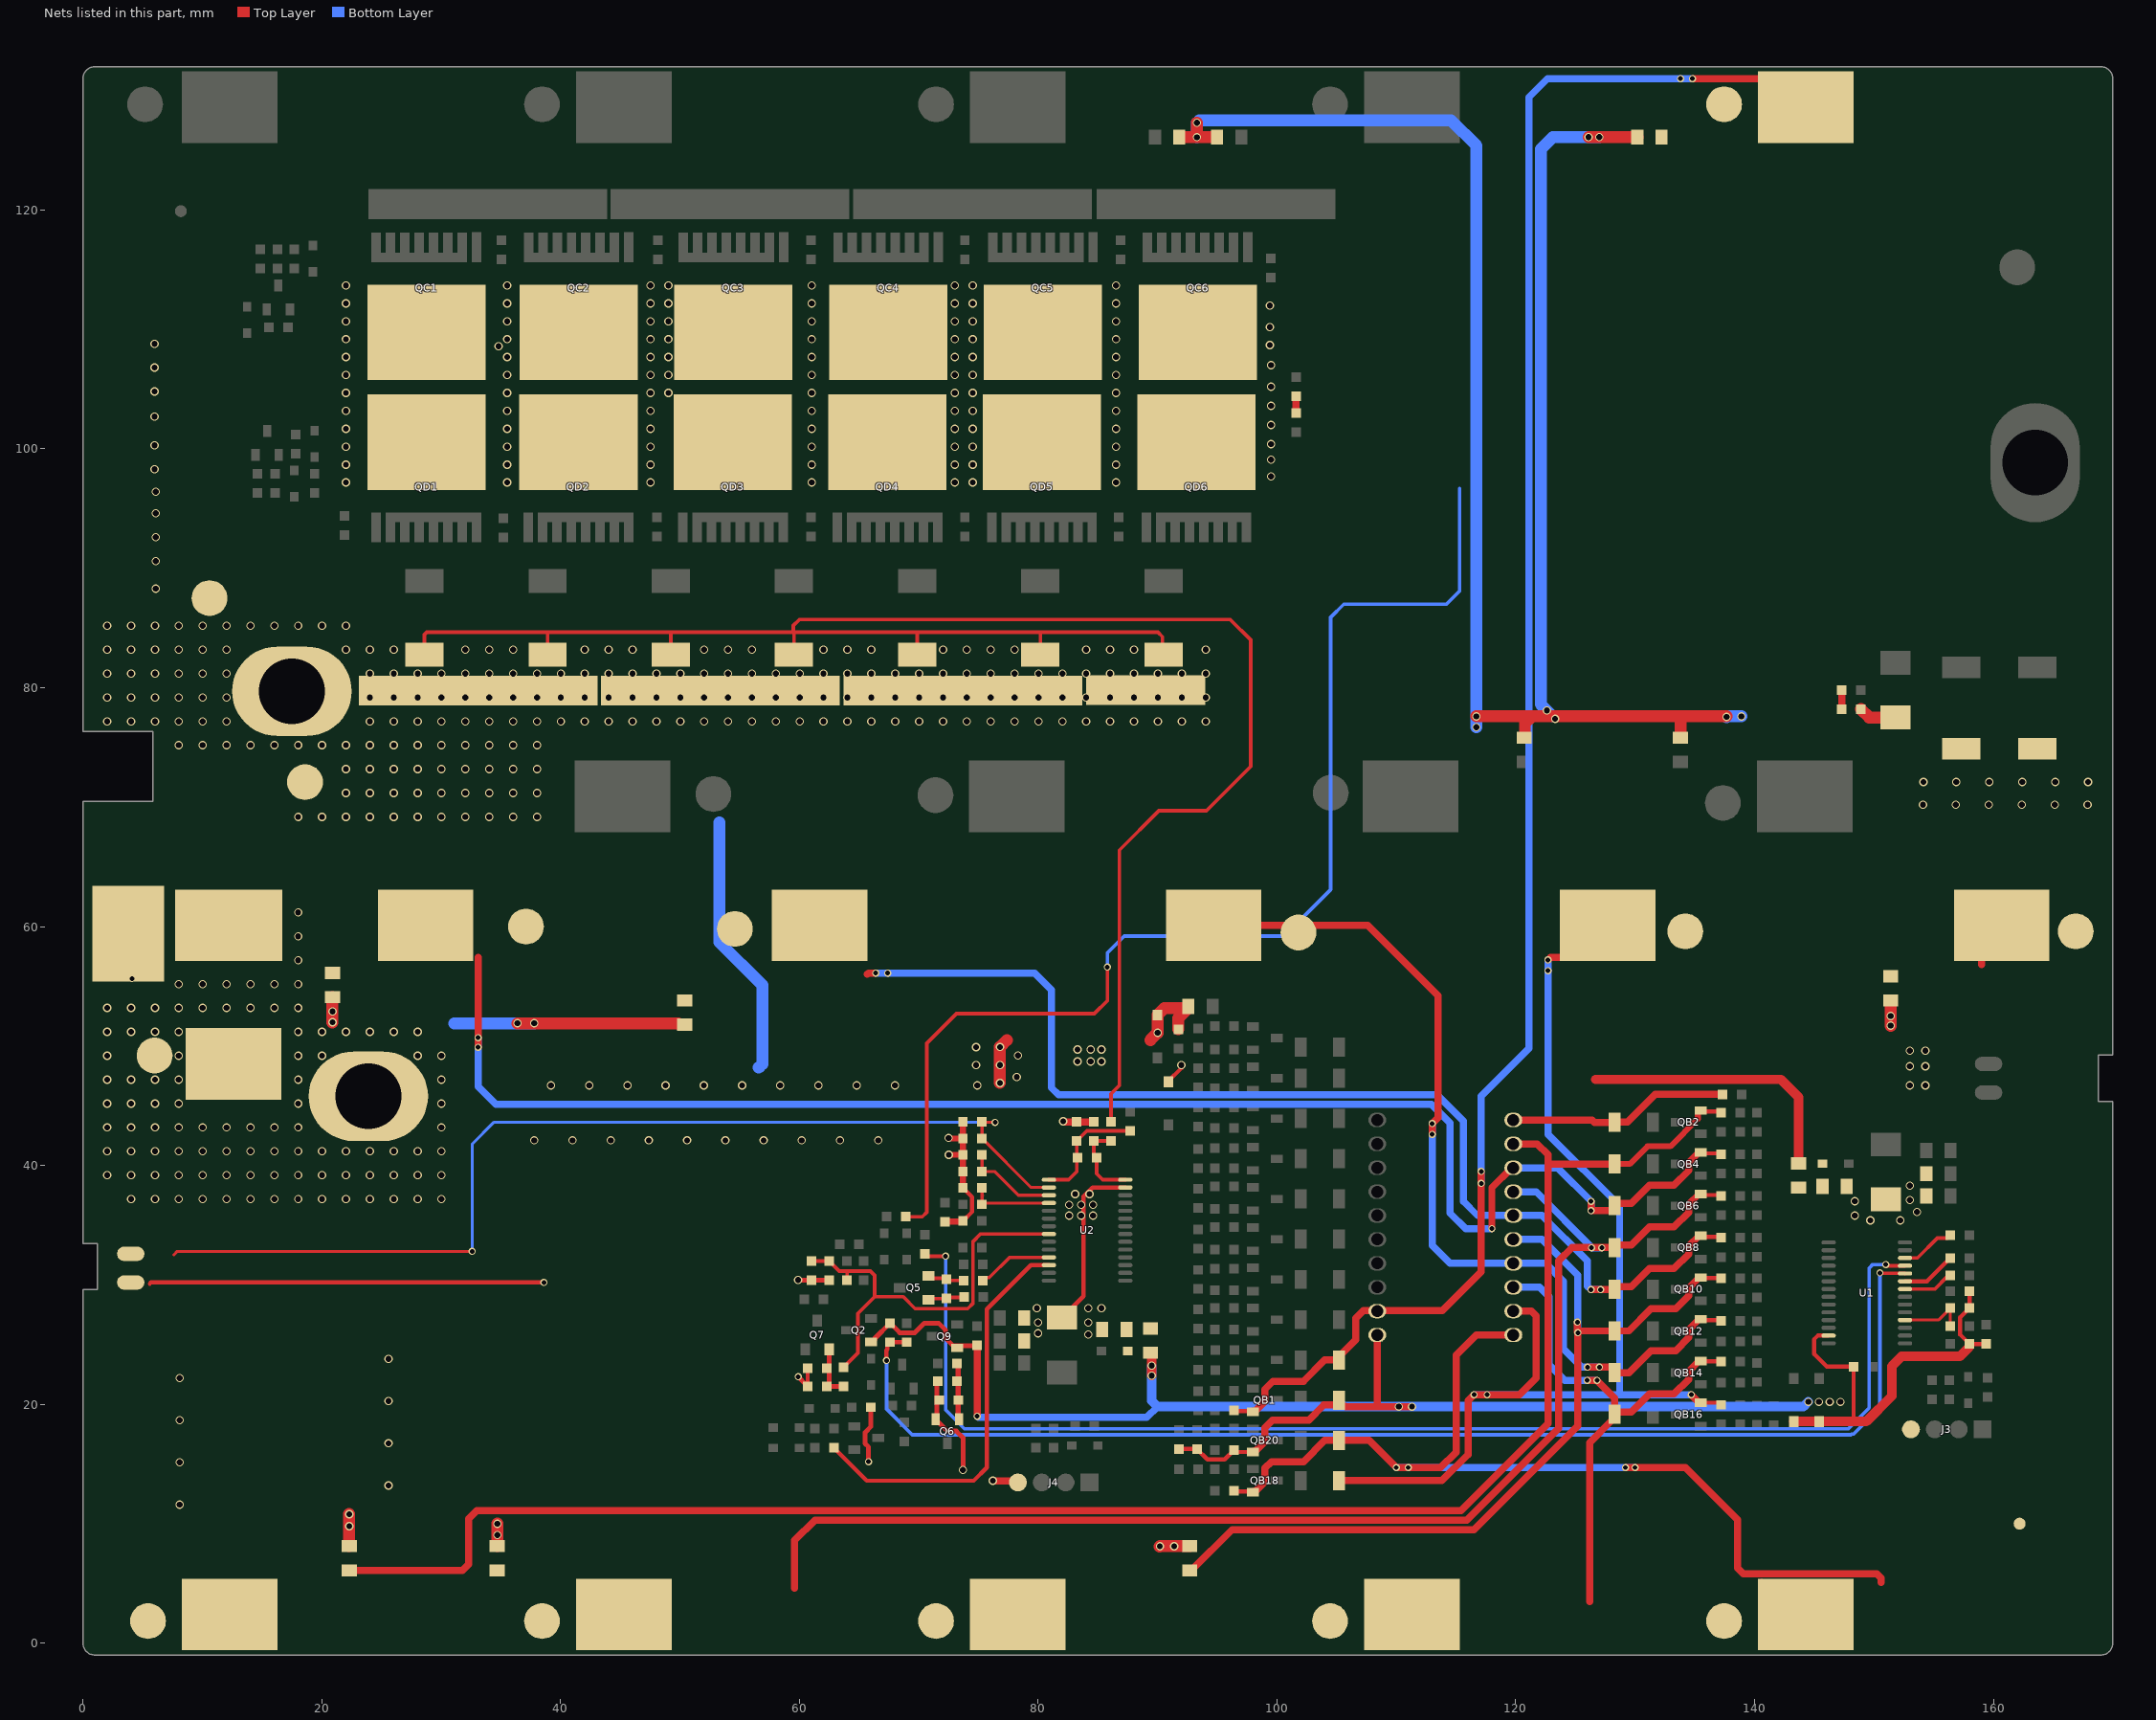
[diagram p0: the nets of this part, all layers, seen from the top]
# Altium PCB MISC82749.PcbDoc (part 2 of 4)
Units mm, origin at the board's own origin, x right, y up, seen from the top; angles counter-clockwise.
Board outline 170 x 133 mm, 2 copper layers (Top Layer, Bottom Layer); 262 components, 170 nets, 783 pads, 1052 vias.

## Via types
v1: diameter 0.7, hole 0.5, Top Layer to Bottom Layer, tented both sides, 953 vias
v2: diameter 0.6, hole 0.4, Top Layer to Bottom Layer, tented both sides, 99 vias

## Nets (pads, with @x,y where several pads share a name; then routed paths per layer and width w, separated by ;. In a path a pad name is that pad's centre, name@x,y a point inside that pad or via, vN(x,y) a via of type N, cw(c..) or ccw(c..) an arc to the next point about the centre after c; other vN are vias at no path point) (continued)
B9: pad.81@144.3,128.6 pad.86@137.45,128.85 pad.89@108.4,27.8 QB1.2 R13.1 RB5.1 RX7.2 | length 153.3
  Top Layer w0.35: R13.1@96.4,19.5 96.465,19.435 97.919,19.435 QB1.2@97.984,19.37
  Top Layer w0.6: QB1.2@97.984,19.37 98.034,19.42 98.184,19.42 99,20.236 99,21.25 99.681,21.931 102.225,21.931 104.007,23.714 RB5.1@105.2,23.714 105.2,24.014 106.6,25.414 106.6,27.2 107.236,27.836 113.836,27.836 117.1,31.1 v2(117.1,38.5) v2(117.1,39.5) ; v2(134.8,131) 141.9,131 pad.81@144.3,128.6
  Bottom Layer w0.6: v2(117.1,38.5) 117.1,45.806 121.1,49.806 121.1,129.45 122.65,131 v2(133.8,131) v2(134.8,131)
B10: C11.1 C23.1 C25.1 C28.1 C36.1 C38.2 D3.2 D6.2 J3.4 pad.75 pad.81@160.7,60.1 pad.86@166.9,59.6 pad.90@108.4,25.8 Q2.1 Q9.1 QB20.2 R11.1 R12.1 R25.2 R28.1 R49.2 R64.2 R71.1 RB1.1 RT5.2 RX6.1 RX7.1 RX8.1 RX9.1 RX10.1 RX11.1 TVS1.2 U1.13 | length 321.5
  Top Layer w0.35: R11.1@91.8,16.25 C11.1@93.3,16.25 94.175,15.375 95.625,15.375 R12.1@96.4,16.15 ; R12.1@96.482,16.232 96.711,16.002 QB20.2@97.984,16.002 ; U1.13@146.2,25.75 145.3,25.75 145,25.45 145,24.2 146.05,23.15 R28.1@148.3,23.15 148.3,18.9 147.95,18.55 ; C36.1@158,29.45 C38.2@158,28.05 157.225,27.275 157.225,25.825 R71.1@158,25.05 RT5.2@159.4,25.05
  Top Layer w0.4: Q2.1@66.025,25.225 66.15,25.225 66.3,25.375 66.3,25.5 R49.2@67.6,26.8 68.4,26 69.671,26 70.471,26.8 71.659,26.8 72.25,26.209 72.25,25.525 72.888,24.888 74.838,24.888 R64.2@74.9,24.95
  Top Layer w0.6: v2(74.9,19) R64.2@74.9,24.95 ; QB20.2@97.984,16.002 98.034,16.052 98.184,16.052 98.984,16.852 98.984,18.034 99.632,18.682 102.682,18.682 103.934,19.934 105,19.934 105.2,20.134 RB1.1@105.2,20.345 105.2,20.045 105.4,19.845 105.706,19.845 105.751,19.8 108.4,19.8 ; pad.90@108.4,25.8 108.4,19.8 ; v1(111.3,19.8) v1(110.2,19.8) 108.4,19.8 ; R71.1@158,24.8 R71.1@158,25.05 ; 159,56.8 pad.81@159,57.35
  Top Layer w0.8: R25.2@89.41,24.31 89.5,24.219 v1(89.5,23.235) v1(89.5,22.4) ; D6.2@143.3,18.55 D3.2@145.4,18.55 147.95,18.55 149.35,18.55 151.5,20.7 151.5,23.193 152.307,24 157.2,24 R71.1@158,24.8
  Top Layer w1: RX11.1@91.816,126.1 93.294,126.1 v1(93.3,126.094) ; v1(93.3,127.3) v1(93.3,126.094) ; RX9.1@94.984,126.1 93.306,126.1 v1(93.3,126.094) ; v1(116.7,77.6) 121.352,77.6 ; RX10.1@120.7,75.816 120.758,75.816 120.766,75.824 120.766,77.014 121.352,77.6 ; v1(126.1,126.1) v1(127,126.1) RX7.1@130.184,126.1 ; RX8.1@133.8,75.816 133.8,77.5 133.9,77.6 ; v1@137.65,77.6 133.9,77.6 ; 121.352,77.6 133.9,77.6
  Bottom Layer w0.6: v2(74.9,19) 75,18.9 89.1,18.9 90,19.8
  Bottom Layer w0.8: v1(89.5,23.235) 89.5,20.3 90,19.8 v1(110.2,19.8) v1(111.3,19.8) 144.1,19.8 v1(144.5,20.2)
  Bottom Layer w1: v1(93.3,126.094) v1(93.3,127.3) 93.5,127.5 114.586,127.5 116.7,125.386 v1(116.7,77.6) v1(116.7,76.7) ; v1@123.1,77.6 122.1,78.6 122.1,125.1 123.1,126.1 v1(126.1,126.1) v1(127,126.1) ; v1(137.65,77.55) 137.7,77.6 v1(138.9,77.6)
  other v1: 145.4,20.2 146.3,20.2 147.2,20.2 149.7,35.4 152.2,35.4 148.4,35.8 153.6,36.1 148.4,37 153,37.1 153,38.3 123.3,77.4 122.6,78.1
B11: pad.81@144.3,2.4 pad.86@137.45,1.85 pad.90@119.8,25.8 QB18.2 R10.1 RB38.1 | length 89
  Top Layer w0.35: R10.1@96.4,12.75 96.458,12.692 97.926,12.692 QB18.2@97.984,12.634
  Top Layer w0.6: QB18.2@97.984,12.634 98.034,12.684 98.184,12.684 99,13.5 99,14.65 99.537,15.187 102.217,15.187 104.007,16.977 RB38.1@105.2,16.977 105.211,16.989 107.711,16.989 v2(110,14.7) v2(111,14.7) 113.7,14.7 115,16 115,24.1 116.7,25.8 pad.90@119.8,25.8 ; v2(129.2,14.7) 134.2,14.7 138.58,10.32 138.58,6.28 139.061,5.8 150.249,5.8 150.6,5.449 150.6,5.1 ; pad.81@140.6,5.1 143.3,2.4 pad.81@144.3,2.4
  Bottom Layer w0.6: v2(110,14.7) v2(111,14.7) v2(129.2,14.7) v2(130,14.7)
B12: pad.81@127.7,60.1 pad.86@134.2,59.6 pad.89@119.8,27.8 QB16.2 R9.1 RB34.1 | length 96.1
  Top Layer w0.35: QB16.2@135.5,20.125 136.957,20.125 R9.1@137.2,19.882
  Top Layer w0.6: RB34.1@105.2,13.609 105.395,13.609 105.4,13.605 113.805,13.605 116,15.8 116,20.3 v2(116.5,20.8) v2(117.6,20.8) 120.3,20.8 121.7,22.2 121.7,27.4 121.3,27.8 pad.89@119.8,27.8 ; v2(122.7,57.2) 122.9,57.4 125,57.4 pad.81@127.7,60.1 ; v2(134.7,20.8) 135.3,20.2 135.3,20.175 135.35,20.125 QB16.2@135.5,20.125
  Bottom Layer w0.6: v2(116.5,20.8) v2(117.6,20.8) 128.7,20.8 ; 122.7,55.9 v2(122.7,57.2) ; 122.719,55.881 122.719,42.6 128.7,36.619 128.7,20.8 ; v2(134.7,20.8) 128.7,20.8
  other v2: 122.7,56.3
B13: pad.81@111.3,2.4 pad.86@104.45,1.85 pad.90@119.8,29.8 QB14.2 R8.1 RB30.1 | length 49.8
  Top Layer w0.35: QB14.2@135.5,23.62 135.524,23.597 137.176,23.597 R8.1@137.2,23.573
  Top Layer w0.6: pad.81@108.351,4.949 pad.81@111.3,2 ; v2(125.987,22) v2(126.805,22) 128.284,20.521 RB30.1@128.284,19.157 ; 126.21,3.471 126.21,16.8 128.06,18.65 128.084,18.65 128.284,18.85 RB30.1@128.284,19.15 RB30.1@128.284,19.157 ; QB14.2@135.5,23.62 135.35,23.62 134.484,22.754 134.484,22.088 133.265,20.869 131.196,20.869 129.684,19.357 128.484,19.357 RB30.1@128.284,19.157
  Bottom Layer w0.6: pad.90@119.8,29.8 122,29.8 122.8,29 122.8,23.3 124.1,22 v2(125.987,22) v2(126.805,22)
B14: pad.81@94.7,60.1 pad.86@101.8,59.5 pad.89@119.8,31.8 QB12.2 R7.1 RB26.1 | length 79
  Top Layer w0.35: QB12.2@135.5,27.116 135.576,27.04 137.124,27.04 R7.1@137.2,26.964
  Top Layer w0.6: pad.81@94.7,60.5 pad.81@94.7,60.1 107.6,60.1 113.5,54.2 113.5,44 v2(113,43.5) v2(113,42.6) ; v2(126,23.1) 128.084,23.1 128.284,22.9 RB26.1@128.284,22.645 129.477,22.645 131.323,24.491 133.392,24.491 134.484,25.584 134.484,26.25 135.35,27.116 QB12.2@135.5,27.116
  Bottom Layer w0.6: v2(113,43.5) v2(113,42.6) 113,33.3 114.5,31.8 pad.89@119.8,31.8 122.5,31.8 124,30.3 124,24.621 125.521,23.1 v2(126,23.1) v2(127,23.1)
B15: pad.81@78.3,2.4 pad.86@71.45,1.85 pad.90@119.8,33.8 QB10.2 R6.1 RB22.1 RX5.2 | length 73.5
  Top Layer w0.35: QB10.2@135.5,30.611 135.528,30.583 137.172,30.583 R6.1@137.2,30.555
  Top Layer w0.6: pad.81@77.2,3.1 pad.81@78.3,2 ; RX5.2@92.7,6.084 92.827,6.084 96.243,9.5 116.5,9.5 125.2,18.2 125.2,21.655 125.187,21.669 125.187,22.331 125.2,22.345 v2(125.2,26) ; v2(125.169,26.869) 125.169,26.031 v2(125.2,26) ; QB10.2@135.5,30.611 135.35,30.611 134.484,29.745 134.484,29.079 133.4,27.995 131.331,27.995 129.477,26.141 RB22.1@128.284,26.141 125.341,26.141 v2(125.2,26)
  Bottom Layer w0.6: pad.90@119.8,33.8 122.2,33.8 125.2,30.8 v2@125.2,26.07
B16: pad.81@61.7,60.1 pad.86@54.6,59.8 pad.90@119.8,35.8 QB8.2 R5.1 RB18.1 RX4.2 | length 95.5
  Top Layer w0.35: QB8.2@135.5,34.106 135.581,34.026 137.119,34.026 R5.1@137.2,33.945
  Top Layer w0.6: 65.7,56 65.8,56.1 v2(66.4,56.1) ; v2(126.3,29.6) RB18.1@128.248,29.6 ; RB18.1@128.3,29.659 128.484,29.843 129.684,29.843 131.196,31.355 133.265,31.355 134.484,32.574 134.484,33.24 135.35,34.106 QB8.2@135.5,34.106
  Bottom Layer w0.6: v2(66.4,56.1) v2(67.4,56.1) 79.7,56.1 81.1,54.7 81.1,46.5 81.7,45.9 113.4,45.9 115.6,43.7 115.6,37 116.8,35.8 pad.90@119.8,35.8 122.2,35.8 126,32 126,29.9 v2(126.3,29.6) v2(127.1,29.6)
B17: pad.81@45.3,2.4 pad.86@38.45,1.85 pad.89@119.8,37.8 QB6.2 R4.1 RB14.1 RX3.2 | length 111.6
  Top Layer w0.35: QB6.2@135.5,37.602 135.583,37.519 137.117,37.519 R4.1@137.2,37.436
  Top Layer w0.6: 59.6,4.6 59.6,8.6 61.3,10.3 115.9,10.3 123.6,18 123.6,32 124.731,33.131 127.169,33.131 v2(127.2,33.1) 127.231,33.131 128.277,33.131 128.484,33.339 129.684,33.339 131.196,34.851 133.265,34.851 134.484,36.07 134.484,36.736 135.35,37.602 QB6.2@135.5,37.602
  Bottom Layer w0.6: pad.89@119.8,37.8 121.7,37.8 126.4,33.1 v2(127.2,33.1)
  other v2: 126.337,33.1
B18: pad.81@28.7,60.1 pad.86@37.1,60 pad.89@119.8,39.8 QB4.2 R3.1 RB10.1 RX2.2 | length 134.6
  Top Layer w0.35: QB4.2@135.5,41.097 135.585,41.012 137.115,41.012 R3.1@137.2,40.927
  Top Layer w0.6: v2(33.1,49.9) v2(33.1,50.7) 33.1,57.4 ; v2(118,34.7) 118,38.15 119.65,39.8 pad.89@119.8,39.8 ; v2(126.3,37) v2(126.3,36.2) 128.084,36.2 128.284,36.4 128.284,36.634 128.484,36.834 129.684,36.834 131.196,38.346 133.265,38.346 134.484,39.565 134.484,40.231 135.35,41.097 QB4.2@135.5,41.097
  Top Layer w1: RX2.2@20.85,56.124 20.858,56.116 RX2.2@20.9,56.116
  Bottom Layer w0.6: v2(33.1,50.7) v2(33.1,49.9) 33.1,46.6 34.6,45.1 112.949,45.1 114.5,43.549 114.5,36 115.8,34.7 v2(118,34.7) ; pad.89@119.8,39.8 123.5,39.8 v2(126.3,37) v2(126.3,36.2)
B19: pad.81@12.3,2.4 pad.86@5.45,1.85 pad.90@119.8,41.8 QB2.2 R2.1 RB6.1 RX1.2 | length 150.3
  Top Layer w0.35: QB2.2@135.5,44.593 135.587,44.505 137.112,44.505 R2.1@137.2,44.418
  Top Layer w0.5: RB6.1@128.284,40.122 129.548,40.122 131.027,41.602 132.955,41.602 135.25,43.897 135.25,44.493 135.35,44.593 QB2.2@135.5,44.593
  Top Layer w0.6: RX1.2@22.3,6.084 31.784,6.084 32.3,6.6 32.3,10.4 33,11.1 115.4,11.1 122.7,18.4 122.7,40.122 122.7,40.9 121.8,41.8 pad.90@119.8,41.8 ; 122.7,40.1 122.722,40.122 RB6.1@128.284,40.122
B+: C40.2 D9.1 pad. pad.66@23.904,45.783 pad.81@3.8,59.4 pad.81@12.2,60.1 pad.81@12.6,48.5 pad.86@6,49.2 R1.1 R24.2 RB2.1 RX1.1 RX2.1 RX3.1 RX4.1 RX5.1 RX6.2 TVS3.2 TVS4.2 | length 76.9
  Top Layer w0.6: pad.@119.8,43.8 126.4,43.8 126.6,43.6 126.609,43.609 128.275,43.609 RB2.1@128.284,43.618 129.368,43.618 131.7,45.95 R1.1@137.3,45.95
  Top Layer w0.8: 126.7,47.2 142.2,47.2 143.7,45.7 R24.2@143.7,40.166
  Top Layer w1: v1(20.9,51.984) v1(20.9,52.884) RX2.1@20.9,54.084 ; RX1.1@22.3,8.116 v1(22.3,10.8) ; RX3.1@34.7,8.116 v1(34.7,9.058) v1(34.7,10) ; v1(36.4,51.9) 49.848,51.9 49.956,51.792 50.392,51.792 RX4.1@50.4,51.784 ; v1@90.184,8.1 90.2,8.116 RX5.1@92.7,8.116 ; C40.2@148.9,78.2 149.6,77.5 D9.1@151.8,77.5 ; v1(151.4,51.7) RX6.2@151.4,53.8
  Bottom Layer w1: 31.1,51.9 v1(36.4,51.9) v1(37.8,51.9)
  other v1: 90.2,8.1 91.4,8.1 22.3,9.8 8.1,11.6 25.6,13.2 8.1,15.133 25.6,16.733 8.1,18.667 25.6,20.267 8.1,22.2 25.6,23.8 4.027,37.182 6.027,37.182 8.027,37.182 10.027,37.182 12.027,37.182 14.027,37.182 16.027,37.182 18.027,37.182 20.027,37.182 22.027,37.182 24.027,37.182 26.027,37.182 28.027,37.182 30.027,37.182 2.027,39.182 4.027,39.182 6.027,39.182 8.027,39.182 10.027,39.182 12.027,39.182 14.027,39.182 16.027,39.182 18.027,39.182 20.027,39.182 22.027,39.182 24.027,39.182 26.027,39.182 28.027,39.182 30.027,39.182 2.027,41.182 4.027,41.182 6.027,41.182 8.027,41.182 10.027,41.182 12.027,41.182 14.027,41.182 16.027,41.182 18.027,41.182 20.027,41.182 22.027,41.182 24.027,41.182 26.027,41.182 28.027,41.182 30.027,41.182 2.027,43.182 4.027,43.182 6.027,43.182 8.027,43.182 10.027,43.182 12.027,43.182 14.027,43.182 16.027,43.182 18.027,43.182 30.027,43.182 2.027,45.182 4.027,45.182 6.027,45.182 8.027,45.182 18.027,45.182 30.027,45.182 153,46.7 154.3,46.7 2.027,47.182 4.027,47.182 6.027,47.182 8.027,47.182 18.027,47.182 30.027,47.182 153,48.3 154.3,48.3 2.027,49.182 8.027,49.182 18.027,49.182 20.027,49.182 28.027,49.182 30.027,49.182 153,49.6 154.3,49.6 2.027,51.182 4.027,51.182 6.027,51.182 8.027,51.182 18.027,51.182 20.027,51.182 22.027,51.182 24.027,51.182 26.027,51.182 28.027,51.182 151.4,52.5 2.027,53.182 4.027,53.182 6.027,53.182 8.027,53.182 10.027,53.182 12.027,53.182 14.027,53.182 16.027,53.182 18.027,53.182 8.027,55.182 10.027,55.182 12.027,55.182 14.027,55.182 16.027,55.182 18.027,55.182 18.027,57.182 18.027,59.182 18.027,61.182 154.1,70.2 156.86,70.2 159.62,70.2 162.38,70.2 165.14,70.2 167.9,70.2 154.14,72.1 156.9,72.1 159.66,72.1 162.42,72.1 165.18,72.1 167.94,72.1
  other v2: 4.1,55.65
CHG_S: R49.1 R59.2 U1.24 | length 105.6
  Top Layer w0.3: v2(150.5,31) 150.54,30.96 152.59,30.96 U1.24@152.6,30.95
  Top Layer w0.35: v2(67.3,23.675) 67.3,24.514 67.375,24.589 67.375,24.975 R49.1@67.6,25.2 R59.2@69,25.2
  Bottom Layer w0.3: v2(67.3,23.675) 67.3,19.6 69.45,17.45 148.057,17.45 148.107,17.5 148.3,17.5 150.5,19.7 v2(150.5,31)
CHGD_M: R57.2 U2.26 | length 34.4
  Top Layer w0.35: R57.2@62.9,16.35 65.65,13.6 74.6,13.6 75.7,14.7 75.7,27.964 79.386,31.65 U2.26@80.9,31.65
CHGD_S: R48.2 U1.26 | length 4.6
  Top Layer w0.3: U1.26@152.6,32.25 153.65,32.25 155.307,33.907 156.157,33.907 R48.2@156.4,34.15
CTLD_M: C47.2 R51.2 R68.1 R69.1 U2.22 | length 36
  Top Layer w0.3: C47.2@61,32 R69.1@62.5,32 63.35,31.15 63.938,31.15 ; R51.2@63.7,23.1 64.9,24.3 64.9,27.6 66.3,29 ; R68.1@64,30.4 64,31.088 63.938,31.15 ; U2.22@80.9,34.25 75.155,34.25 74.55,33.645 74.55,31.05 74.55,28.455 74.095,28 69.7,28 68.7,29 66.3,29 ; 63.938,31.15 65.945,31.15 66.3,30.795 66.3,29
CTLD_S: R31.2 U1.22 | length 3.9
  Top Layer w0.3: U1.22@152.6,29.65 155.1,29.65 R31.2@156.117,30.667
DSG_S: R44.2 U1.23 | length 4.6
  Top Layer w0.35: U1.23@152.6,30.3 154.45,30.3 R44.2@156.4,32.25
DSGD_M: R46.2 U2.25 | length 6.3
  Top Layer w0.3: R46.2@75.36,30.36 75.61,30.61 75.91,30.61 77.6,32.3 U2.25@80.9,32.3
DSGD_S: R55.2 U1.25 | length 108.3
  Top Layer w0.3: R55.2@70.5,32.6 70.7,32.4 v2(72.25,32.4) ; v2(151,31.7) 151.081,31.7 151.181,31.6 U1.25@152.6,31.6
  Bottom Layer w0.3: v2(72.25,32.4) 72.25,19.522 73.822,17.95 147.85,17.95 149.6,19.7 149.6,31.4 149.9,31.7 v2(151,31.7)
GND: C22.1 C24.1 C26.1 C27.2 C29.1 C31.1 C33.2 C34.1 C37.2 C39.2 C43.1 C44.2 C47.1 D4.2 D5.2 J4.4 NTC2.2 pad.66@17.5,79.7 pad.82@33.1,79.75 pad.83@53.4,79.75 pad.83@73.7,79.75 pad.83@89,79.8 pad.86@10.6,87.5 pad.86@18.6,72.1 Q6.2 R23.1 R29.1 R45.1 R60.1 R63.2 R69.2 RS1.1 RS2.1 RS3.1 RS4.1 RS5.1 RS6.1 RS7.1 RT2.2 RT4.2 RT6.2 TVS2.2 U2.13 | length 282
  Top Layer w0.3: RS7.1@28.6,82.75 28.6,84.445 28.805,84.65 39.053,84.65 ; RS6.1@38.917,82.75 38.917,84.514 39.053,84.65 ; RS5.1@49.233,82.75 49.233,84.583 49.3,84.65 ; RS4.1@59.55,82.75 59.55,84.6 59.5,84.65 ; RS3.1@69.867,82.75 69.867,84.517 70,84.65 ; RS2.1@80.183,82.75 80.183,84.633 80.2,84.65 ; R29.1@86.1,43.65 86.1,46 86.8,46.7 86.8,66.4 90.1,69.7 94.1,69.7 97.8,73.4 97.8,84 96.1,85.7 59.994,85.7 59.5,85.206 59.5,84.65 ; RS1.1@90.5,82.75 90.407,82.843 90.407,84.272 90.03,84.65 80.2,84.65 ; 39.053,84.65 49.3,84.65 ; 49.3,84.65 59.5,84.65 ; 59.5,84.65 70,84.65 ; 70,84.65 80.2,84.65
  Top Layer w0.35: 5.6,30.1 5.7,30.2 v2(38.6,30.2) ; R60.1@60.7,21.5 C44.2@60.7,23 ; C34.1@73.7,35.34 74.475,36.115 74.475,37.345 C39.2@73.7,38.12 ; TVS2.2@82,27.25 83.8,29.05 83.8,37.4 84.55,38.15 U2.13@87.3,38.15 ; C27.2@84.667,43.65 C27.2@84.828,43.65 ; D5.2@90.9,47 90.9,47.05 92,48.15 v1(92,48.4) ; C22.1@91.75,51.4 C22.1@91.808,51.458
  Top Layer w0.4: v2(59.9,22.3) 60.159,22.041 R60.1@60.7,21.5 ; v1(59.9,30.4) C47.1@61,30.4 R69.2@62.5,30.4 ; v2(65.8,15.2) 65.8,16.416 65.5,16.716 65.5,17.634 66,18.134 R45.1@66,19.75 ; R63.2@71.6,21.95 71.513,21.863 71.513,18.838 Q6.2@71.425,18.75 71.425,18.6 71.575,18.45 71.7,18.45 72.4,17.75 73.15,17.75 73.7,17.2 v1(73.7,14.5)
  Top Layer w0.5: RT6.2@72.225,35.305 73.665,35.305 C34.1@73.7,35.34 ; v1(72.5,42.3) 72.54,42.26 RT2.2@73.7,42.26 ; v1(72.52,40.88) RT4.2@73.7,40.88 ; C39.2@73.7,38.12 C37.2@73.7,39.5 RT4.2@73.7,40.88 ; C33.2@73.7,43.64 RT2.2@73.7,42.26 ; RT4.2@73.7,40.88 RT2.2@73.7,42.26
  Top Layer w0.6: v1(76.2,13.6) 76.219,13.581 78.169,13.581 J4.4@78.3,13.45 ; v1(82.1,43.699) 82.127,43.699 82.176,43.65 C31.1@83.233,43.65 C27.2@84.667,43.65
  Top Layer w1: v1(76.8,46.9) v1(76.8,49.914) 77.386,50.5 ; 89.4,50.5 v1(90,51.1) D4.2@90,52.6 90.576,53.176 92.581,53.176 92.584,53.173 91.75,52.339 C22.1@91.75,51.4
  Bottom Layer w1: 53.3,68.7 53.3,58.7 56.9,55.1 56.9,48.5 56.6,48.2
  other v1: 84.2,25.85 80,25.95 80,26.85 84.2,26.85 79.9,28.05 84.2,28.05 85.3,28.05 82.6,35.8 83.6,35.8 84.6,35.8 82.6,36.7 83.6,36.7 84.6,36.7 83.1,37.6 84.3,37.6 37.8,42.1 41,42.1 44.2,42.1 47.4,42.1 50.6,42.1 53.8,42.1 57,42.1 60.2,42.1 63.4,42.1 66.6,42.1 39.2,46.7 42.4,46.7 45.6,46.7 48.8,46.7 52,46.7 55.2,46.7 58.4,46.7 61.6,46.7 64.8,46.7 68,46.7 74.9,46.7 78.2,47.4 74.8,48.4 76.8,48.407 83.3,48.7 84.4,48.7 85.3,48.7 78.3,49.2 83.3,49.7 84.4,49.7 85.3,49.7 74.8,49.9 18.027,69.182 20.027,69.182 22.027,69.182 24.027,69.182 26.027,69.182 28.027,69.182 30.027,69.182 32.028,69.182 34.028,69.182 36.028,69.182 38.028,69.182 22.027,71.182 24.027,71.182 26.027,71.182 28.027,71.182 30.027,71.182 32.028,71.182 34.028,71.182 36.028,71.182 38.028,71.182 22.027,73.182 24.027,73.182 26.027,73.182 28.027,73.182 30.027,73.182 32.028,73.182 34.028,73.182 36.028,73.182 38.028,73.182 8.027,75.182 10.027,75.182 12.027,75.182 14.027,75.182 16.027,75.182 18.027,75.182 20.027,75.182 22.027,75.182 24.027,75.182 26.027,75.182 28.027,75.182 30.027,75.182 32.028,75.182 34.028,75.182 36.028,75.182 38.028,75.182 2.027,77.182 4.027,77.182 6.027,77.182 8.027,77.182 10.027,77.182 12.027,77.182 24.027,77.182 26.027,77.182 28.027,77.182 30.027,77.182 32.028,77.182 34.028,77.182 36.028,77.182 38.028,77.182 40.028,77.182 42.028,77.182 44.028,77.182 46.028,77.182 48.028,77.182 50.028,77.182 52.028,77.182 54.028,77.182 56.028,77.182 58.028,77.182 60.028,77.182 62.028,77.182 64.028,77.182 66.028,77.182 68.028,77.182 70.028,77.182 72.028,77.182 74.028,77.182 76.028,77.182 78.028,77.182 80.028,77.182 82.028,77.182 84.028,77.182 86.028,77.182 88.028,77.182 90.028,77.182 92.028,77.182 94.028,77.182 2.027,79.182 4.027,79.182 6.027,79.182 8.027,79.182 10.027,79.182 12.027,79.182 24.027,79.182 26.027,79.182 28.027,79.182 30.027,79.182 32.028,79.182 34.028,79.182 36.028,79.182 38.028,79.182 40.028,79.182 42.028,79.182 44.028,79.182 46.028,79.182 48.028,79.182 50.028,79.182 52.028,79.182 54.028,79.182 56.028,79.182 58.028,79.182 60.028,79.182 62.028,79.182 64.028,79.182 66.028,79.182 68.028,79.182 70.028,79.182 72.028,79.182 74.028,79.182 76.028,79.182 78.028,79.182 80.028,79.182 82.028,79.182 84.028,79.182 86.028,79.182 88.028,79.182 90.028,79.182 92.028,79.182 94.028,79.182 2.027,81.182 4.027,81.182 6.027,81.182 8.027,81.182 10.027,81.182 12.027,81.182 24.027,81.182 26.027,81.182 28.027,81.182 30.027,81.182 32.028,81.182 34.028,81.182 36.028,81.182 38.028,81.182 40.028,81.182 42.028,81.182 44.028,81.182 46.028,81.182 48.028,81.182 50.028,81.182 52.028,81.182 54.028,81.182 56.028,81.182 58.028,81.182 60.028,81.182 62.028,81.182 64.028,81.182 66.028,81.182 68.028,81.182 70.028,81.182 72.028,81.182 74.028,81.182 76.028,81.182 78.028,81.182 80.028,81.182 82.028,81.182 84.028,81.182 86.028,81.182 88.028,81.182 90.028,81.182 92.028,81.182 94.028,81.182 2.027,83.182 4.027,83.182 6.027,83.182 8.027,83.182 10.027,83.182 12.027,83.182 22.027,83.182 24.027,83.182 26.027,83.182 32.028,83.182 34.028,83.182 36.028,83.182 42.028,83.182 44.028,83.182 46.028,83.182 52.028,83.182 54.028,83.182 56.028,83.182 62.028,83.182 64.028,83.182 66.028,83.182 72.028,83.182 74.028,83.182 76.028,83.182 78.028,83.182 84.028,83.182 86.028,83.182 88.028,83.182 94.028,83.182 2.027,85.182 4.027,85.182 6.027,85.182 8.027,85.182 10.027,85.182 12.027,85.182 14.027,85.182 16.027,85.182 18.027,85.182 20.027,85.182 22.027,85.182 6.1,88.3 6.1,90.6 6.1,92.6 6.1,94.6 6.1,96.4 6,98.3 6,100.3 6,102.7 6,104.8 6,106.8 6,108.8
MSO_D-: QC1.3 QC2.3 QC3.3 QC4.3 QC5.3 QC6.3 QD1.3 QD2.3 QD3.3 QD4.3 QD5.3 QD6.3 R66.1 | length 101.5
  Top Layer w0.3: QD1.3@28.01,100 QD1.3@28.56,100.55 ; R66.1@68.9,35.7 70.3,35.7 70.675,36.075 70.675,50.217 73.158,52.7 84.7,52.7 85.8,53.8 v2(85.8,56.6)
  Bottom Layer w0.3: v2(85.8,56.6) 85.8,57.8 87.2,59.2 100.6,59.2 104.5,63.1 104.5,85.9 105.6,87 114.2,87 115.3,88.1 115.3,96.7
  other v1: 22.027,97.182 35.527,97.182 47.527,97.182 61.027,97.182 73.027,97.182 74.527,97.182 86.527,97.182 99.5,97.7 22.027,98.682 35.527,98.682 47.527,98.682 61.027,98.682 73.027,98.682 74.527,98.682 86.527,98.682 99.5,99.1 22.027,100.182 35.527,100.182 47.527,100.182 61.027,100.182 73.027,100.182 74.527,100.182 86.527,100.182 99.5,100.4 22.027,101.682 35.527,101.682 47.527,101.682 61.027,101.682 73.027,101.682 74.527,101.682 86.527,101.682 99.5,102 22.027,103.182 35.527,103.182 47.527,103.182 61.027,103.182 73.027,103.182 74.527,103.182 86.527,103.182 99.5,103.6 22.027,104.682 35.527,104.682 47.527,104.682 49.027,104.682 61.027,104.682 73.027,104.682 74.527,104.682 86.527,104.682 99.5,105.2 22.027,106.182 35.527,106.182 47.527,106.182 49.027,106.182 61.027,106.182 73.027,106.182 74.527,106.182 86.527,106.182 99.5,107 22.027,107.682 35.527,107.682 47.527,107.682 49.027,107.682 61.027,107.682 73.027,107.682 74.527,107.682 86.527,107.682 34.8,108.6 99.4,108.7 22.027,109.182 35.527,109.182 47.527,109.182 49.027,109.182 61.027,109.182 73.027,109.182 74.527,109.182 86.527,109.182 99.4,110.2 22.027,110.682 35.527,110.682 47.527,110.682 49.027,110.682 61.027,110.682 73.027,110.682 74.527,110.682 86.527,110.682 99.4,112 22.027,112.182 35.527,112.182 47.527,112.182 49.027,112.182 61.027,112.182 73.027,112.182 74.527,112.182 86.527,112.182 22.027,113.682 35.527,113.682 47.527,113.682 49.027,113.682 61.027,113.682 73.027,113.682 74.527,113.682 86.527,113.682
NetC23_2: C23.2 D1.2 R24.1
NetC24_2: C24.2 D2.2 R25.1
NetC27_1: C27.1 C30.2 R29.2 U2.14 | length 6.8
  Top Layer w0.3: C30.2@84.667,40.65 C27.1@84.667,42.05 R29.2@86.1,42.05 ; C30.2@84.9,40.65 84.9,39.3 85.4,38.8 U2.14@87.3,38.8
NetC30_1: C30.1 C31.2 R30.1 U2.15 | length 10
  Top Layer w0.3: U2.15@80.9,38.8 82.558,38.8 83.233,39.475 C31.2@83.233,42.05 84.083,42.9 R30.1@87.7,42.9
NetC33_1: C33.1 NTC2.1 RT2.1 U2.16 | length 88.5
  Top Layer w0.25: NTC2.1@4,32.6 NTC2.1@4.002,32.598 ; 7.6,32.5 7.9,32.8 v2(32.6,32.8) ; v2(76.4,43.6) 75.34,43.6 C33.1@75.3,43.64 RT2.1@75.3,42.26 79.41,38.15 U2.16@80.9,38.15
  Bottom Layer w0.25: v2(32.6,32.8) 32.6,41.8 34.4,43.6 v2(76.4,43.6)
NetC37_1: C37.1 RT4.1 U2.17 | length 7.8
  Top Layer w0.25: RT4.1@75.3,40.88 C37.1@75.3,39.5 76.35,39.5 78.35,37.5 U2.17@80.9,37.5
NetC38_1: C38.1 RT7.2 U1.18 | length 5.7
  Top Layer w0.25: U1.18@152.6,27.05 155.4,27.05 C38.1@156.4,28.05 RT7.2@156.4,26.55
NetC39_1: C39.1 RT8.2 U2.18 | length 7
  Top Layer w0.25: RT8.2@75.3,36.74 75.3,37.52 ; C39.1@75.3,38.12 75.3,37.52 ; 75.35,37.47 75.3,37.52 ; RT8.2@75.359,36.85 U2.18@80.9,36.85
NetC40_1: C40.1 C41.2 | length 1.6
  Top Layer w0.6: C40.1@147.3,78.2 C41.2@147.3,79.8
NetC42_1: C42.1 Q5.1 R47.1 | length 3.1
  Top Layer w0.3: Q5.1@70.8,28.55 71.1,28.85 C42.1@72.3,28.85 ; C42.1@72.3,28.95 R47.1@73.8,28.95
NetC42_2: C42.2 Q5.2 R46.1 | length 2.7
  Top Layer w0.3: Q5.2@71.095,30.555 72.195,30.555 C42.2@72.3,30.45 ; C42.2@72.3,30.36 R46.1@73.76,30.36
NetC43_2: C43.2 Q6.1 R62.1 R63.1 | length 4.8
  Top Layer w0.45: R62.1@73.2,23.45 73.288,23.363 73.288,21.95 73.288,20.35 73.288,18.838 Q6.1@73.375,18.75
NetC44_1: C44.1 Q7.2 R51.1 R60.2 | length 4.7
  Top Layer w0.4: Q7.2@62.5,24.6 62.5,23.2 C44.1@62.3,23 62.5,22.8 62.5,21.7 R60.2@62.3,21.5 62.5,21.5 R51.1@63.7,21.5
NetC45_1: C45.1 C46.2 | length 1.4
  Top Layer w0.6: C45.1@101.6,103 C46.2@101.6,104.4